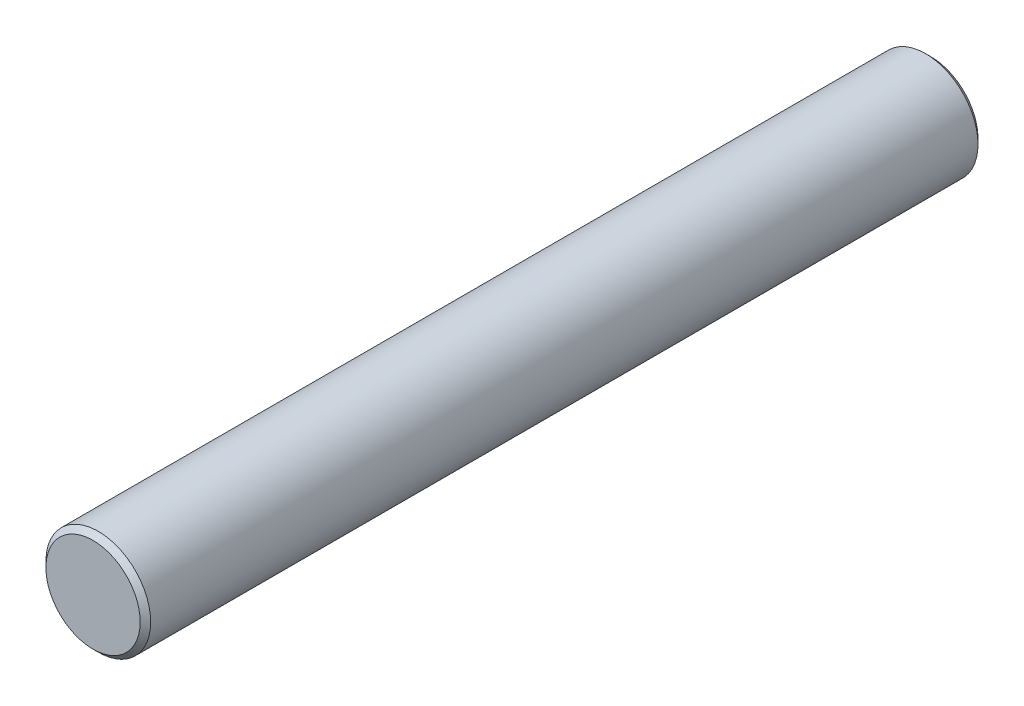
from build123d import *

# Parameters (mm, degrees)
SKETCH_1_R      = 5
EXTRUDE_1_DEPTH = 80
CHAMFER_1_SIZE  = 0.5


with BuildPart() as part:
    # 草图1 → 凸台-拉伸1 (new body)
    with BuildSketch(Plane.XY):
        Circle(SKETCH_1_R)
    extrude(amount=EXTRUDE_1_DEPTH)

    # 倒角1
    chamfer_1_edges = [part.edges().sort_by_distance(p)[0] for p in [
        (-5, 0, 0),
        (-5, 0, 80),
    ]]
    chamfer(chamfer_1_edges, length=CHAMFER_1_SIZE)


solid = part.part
